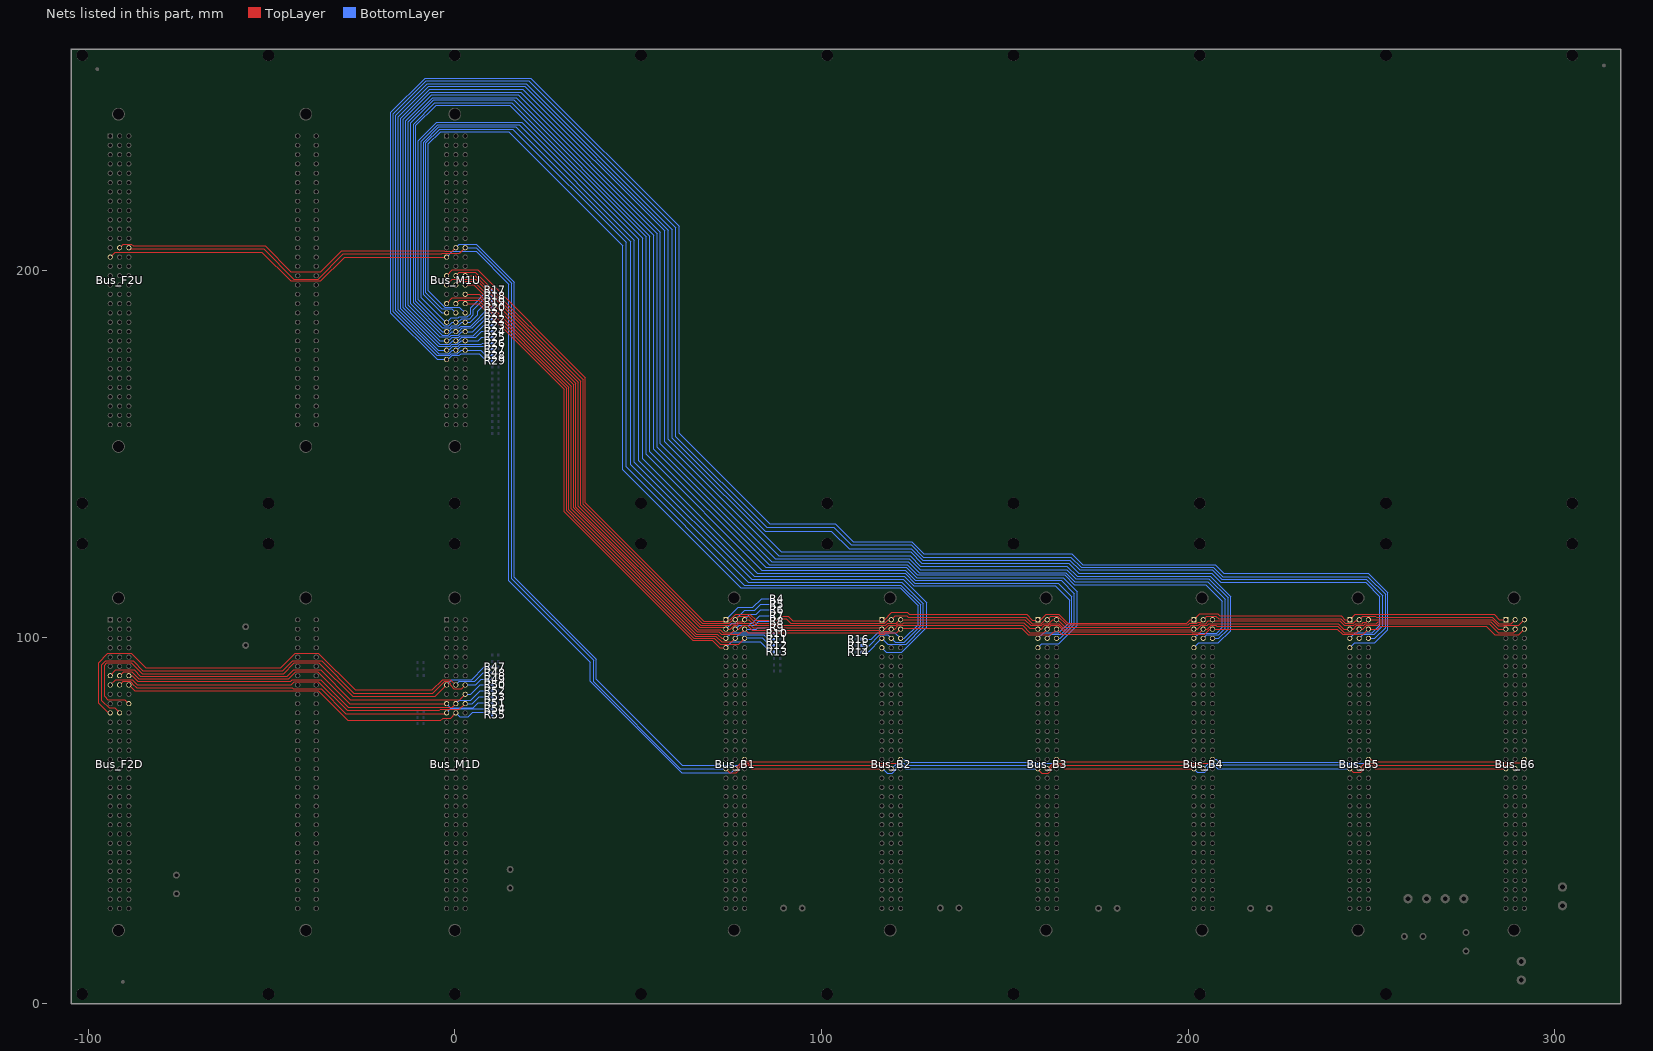
[diagram p0: the nets of this part, all layers, seen from the top]
# Altium PCB MISC67337.PcbDoc (part 6 of 7)
Units mm, origin at the board's own origin, x right, y up, seen from the top; angles counter-clockwise.
Board outline 422.71 x 260.35 mm, 4 copper layers (TopLayer, InternalPlane1, InternalPlane2, BottomLayer); 82 components, 143 nets, 1295 pads, 42 vias.

## Via types
v1: diameter 0.61, hole 0.305, TopLayer to BottomLayer, 42 vias

## Nets (pads, with @x,y where several pads share a name; then routed paths per layer and width w, separated by ;. In a path a pad name is that pad's centre, name@x,y a point inside that pad or via, vN(x,y) a via of type N, cw(c..) or ccw(c..) an arc to the next point about the centre after c; other vN are vias at no path point) (continued)
B_DSP2_XD13: Bus_B1.C16 Bus_B2.C16 Bus_B3.C16 Bus_B4.C16 Bus_B5.C16 Bus_B6.C16 Bus_F2U.B13 Bus_M1U.B13 | length 511.1
  TopLayer w0.254: Bus_F2U.B13@-91.388,206.173 Bus_F2U.B13@-91.43,206.173 -90.466,207.137 -90.272,207.137 -90.257,207.151 -88.203,207.151 -87.74,206.688 -54.813,206.688 ; -54.102,206.688 -54.813,206.688 ; -29.5,205.327 -28.956,205.327 ; Bus_M1U.B13@0.3,206.173 -0.678,205.196 -2.732,205.196 -2.863,205.327 -28.956,205.327 ; Bus_B1.C16@79.035,66.504 79.144,66.504 79.683,65.965 107.848,65.965 ; 110.425,65.965 107.848,65.965 ; Bus_B2.C16@121.585,66.613 120.504,65.532 115.773,65.532 115.34,65.965 107.848,65.965 ; Bus_B3.C16@164.13,66.613 165.01,66.613 165.653,65.97 200.476,65.97 200.889,65.557 ; 200.863,65.557 200.889,65.557 ; Bus_B4.C16@206.675,66.486 205.746,65.557 200.889,65.557 ; Bus_B5.C16@249.22,66.613 249.885,66.613 250.52,65.978 252.552,65.978 ; 251.079,65.978 252.552,65.978 ; 278.638,65.978 277.241,65.978 ; Bus_B6.C16@291.765,66.613 290.787,65.635 285.75,65.635 285.407,65.978 277.241,65.978 ; -54.813,206.688 -51.723,206.688 -44.679,199.644 -36.5,199.644 -30.817,205.327 -28.956,205.327 ; 252.552,65.978 277.241,65.978
  BottomLayer w0.254: Bus_M1U.B13@0.3,206.173 1.278,207.151 5.904,207.151 16.256,196.799 16.256,116.332 38.608,93.98 38.608,88.519 62.076,65.051 77.473,65.051 Bus_B1.C16@79.035,66.613 ; Bus_B2.C16@121.585,66.613 122.617,66.613 123.325,65.905 154.559,65.905 ; 154.813,65.905 154.559,65.905 ; Bus_B3.C16@164.257,66.675 163.176,65.594 160.833,65.594 160.807,65.619 158.318,65.619 158.033,65.905 154.559,65.905 ; Bus_B4.C16@206.675,66.613 207.631,66.613 208.347,65.897 210.947,65.897 ; 210.972,65.897 243.018,65.897 243.357,65.557 245.77,65.557 ; 245.796,65.532 248.139,65.532 Bus_B5.C16@249.22,66.613
B_DSP2_XD14: Bus_B1.A17 Bus_B2.A17 Bus_B3.A17 Bus_B4.A17 Bus_B5.A17 Bus_B6.A17 Bus_F2U.C13 Bus_M1U.C13 | length 508.7
  TopLayer w0.254: Bus_F2U.C13@-88.89,205.833 -53.823,205.833 ; -52.63,205.833 -53.823,205.833 ; -28.637,204.48 -26.518,204.48 ; 1.456,204.789 Bus_M1U.C13@2.84,206.173 1.278,204.611 -3.476,204.611 -3.607,204.48 -26.518,204.48 ; Bus_B1.A17@73.96,64.073 75.041,62.992 76.802,62.992 77.478,63.668 77.478,64.27 78.334,65.126 79.908,65.126 80.961,64.073 Bus_B2.A17@116.505,64.073 ; Bus_B3.A17@159.05,63.946 160.131,62.865 161.892,62.865 162.568,63.541 162.568,64.143 163.525,65.1 165.303,65.1 166.33,64.073 Bus_B4.A17@201.595,64.073 ; Bus_B5.A17@244.14,64.073 245.118,63.095 247.118,63.095 248.031,64.008 248.031,64.389 248.693,65.051 250.087,65.051 251.065,64.073 Bus_B6.A17@286.685,64.073 ; -53.823,205.833 -52.163,205.833 -43.942,197.612 -37.236,197.612 -30.368,204.48 -26.518,204.48
  BottomLayer w0.254: Bus_M1U.C13@2.84,206.173 2.892,206.121 5.893,206.121 15.494,196.52 15.494,115.951 37.846,93.599 37.846,87.757 61.53,64.073 Bus_B1.A17@73.955,64.073 ; Bus_B2.A17@116.632,64.135 117.902,62.865 119.318,62.865 120.396,63.943 120.396,64.451 121.058,65.113 121.933,65.113 122.973,64.073 127.686,64.073 ; 126.467,64.073 127.686,64.073 ; Bus_B3.A17@159.05,64.073 127.686,64.073 ; Bus_B3.A17@159.05,64.116 159.158,64.116 Bus_B3.A17@159.177,64.135 ; Bus_B4.A17@201.595,64.073 202.573,63.095 204.573,63.095 205.359,63.881 205.359,64.389 206.021,65.051 207.161,65.051 208.139,64.073 Bus_B5.A17@244.14,64.073 Bus_B5.A17@244.121,64.054
B_DSP2_XD15: Bus_B1.B17 Bus_B2.B17 Bus_B3.B17 Bus_B4.B17 Bus_B5.B17 Bus_B6.B17 Bus_F2U.A14 Bus_M1U.A14 | length 507.2
  TopLayer w0.254: Bus_F2U.A14@-93.97,203.633 -92.625,204.978 -52.578,204.978 -44.704,197.104 -36.525,197.104 -29.996,203.633 Bus_M1U.A14@-2.24,203.633 ; Bus_B1.B17@76.495,64.073 77.954,65.532 80.077,65.532 80.558,65.051 118.067,65.051 Bus_B2.B17@119.045,64.073 ; Bus_B3.B17@161.59,63.946 163.201,65.557 165.421,65.557 165.927,65.051 203.157,65.051 Bus_B4.B17@204.135,64.073 ; Bus_B4.B17@204.071,64.01 Bus_B4.B17@204.135,63.946 ; Bus_B5.B17@246.68,64.073 248.139,65.532 250.444,65.532 250.951,65.025 277.343,65.025 277.368,65.051 288.247,65.051 Bus_B6.B17@289.225,64.073
  BottomLayer w0.254: Bus_M1U.A14@-2.24,203.633 -0.678,205.196 5.802,205.196 14.732,196.266 14.732,115.316 36.957,93.091 36.957,87.884 61.849,62.992 75.414,62.992 Bus_B1.B17@76.495,64.073 ; Bus_B2.B17@119.172,64.135 120.631,65.594 122.442,65.594 123.047,64.989 154.788,64.989 ; 155.321,64.989 154.788,64.989 ; Bus_B3.B17@161.717,64.135 160.639,65.213 158.013,65.213 157.789,64.989 154.788,64.989 ; Bus_B4.B17@204.135,64.073 205.619,65.557 207.721,65.557 208.128,65.151 245.602,65.151 Bus_B5.B17@246.68,64.073
B_LZL1: Bus_F2D.B11 Bus_M1D.C8 R49.2 | length 132.2
  TopLayer w0.254: Bus_F2D.B11@-91.43,79.294 -92.781,80.645 -94.234,80.645 -96.266,82.677 -96.266,92.456 -95.25,93.472 -87.732,93.472 -85.09,90.83 -46.888,90.83 -44.247,93.472 -36.322,93.472 -27.483,84.633 -6.02,84.633 -2.761,87.892 -1.835,87.892 -1.262,87.319 -1.262,86.987 -0.211,85.936 1.862,85.936 Bus_M1D.C8@2.84,86.914
  BottomLayer w0.254: Bus_M1D.C8@2.84,86.914 5.71,86.914 7.29,88.494 R49.2@10.185,88.494
B_LZL2: Bus_F2D.A11 Bus_M1D.B8 R48.1 | length 134.4
  TopLayer w0.254: Bus_F2D.A11@-93.97,79.294 -94.534,79.294 -97.155,81.915 -97.155,92.964 -94.607,95.512 -88.29,95.512 -84.345,91.567 -47.523,91.567 -43.459,95.631 -37.186,95.631 -27.102,85.547 -6.096,85.547 -3.251,88.392 -1.178,88.392 Bus_M1D.B8@0.3,86.914
  BottomLayer w0.254: Bus_M1D.B8@0.3,86.914 1.278,87.892 5.444,87.892 7.747,90.195 R48.1@10.185,90.195
B_LZL3: Bus_F2D.C10 Bus_M1D.A8 R47.2 | length 131.5
  TopLayer w0.254: Bus_F2D.C10@-88.89,81.834 -89.987,82.931 -94.615,82.931 -95.504,83.82 -95.504,92.329 -94.861,92.972 -88.222,92.972 -85.293,90.043 -46.693,90.043 -43.764,92.972 -37.041,92.972 -27.864,83.795 -5.359,83.795 Bus_M1D.A8@-2.24,86.914
  BottomLayer w0.254: Bus_M1D.A8@-2.24,86.914 -0.762,88.392 4.674,88.392 8.103,91.821 R47.2@10.185,91.821
B_LZT1: Bus_F2D.C8 Bus_M1D.B11 R55.1 | length 105.1
  TopLayer w0.254: Bus_F2D.C8@-88.89,86.914 -87.32,85.344 -37.287,85.344 -29.235,77.292 -3.759,77.292 -3.2,77.851 -1.143,77.851 Bus_M1D.B11@0.3,79.294
  BottomLayer w0.254: Bus_M1D.B11@0.3,79.294 1.362,78.232 3.658,78.232 4.089,78.664 4.115,78.664 4.928,79.477 9.373,79.477 10.084,78.765 R55.1@10.185,78.765
B_LZT2: Bus_F2D.B8 Bus_M1D.A11 R54.2 | length 106.2
  TopLayer w0.254: Bus_F2D.B8@-91.43,86.914 -90.452,87.892 -88.485,87.892 -87.912,87.319 -87.912,87.302 -86.741,86.131 -44.323,86.131 -44.044,85.852 -36.449,85.852 -29.693,79.096 -2.764,79.096 -2.565,79.294 Bus_M1D.A11@-2.24,79.294
  BottomLayer w0.254: Bus_M1D.A11@-2.24,79.294 -1.168,80.366 10.16,80.366 R54.2@10.185,80.391
B_LZT3: Bus_F2D.A8 Bus_M1D.C10 R53.2 | length 110.5
  TopLayer w0.254: Bus_F2D.A8@-93.97,86.914 -92.492,88.392 -87.986,88.392 -86.614,87.02 -44.602,87.02 -43.794,87.828 -37.206,87.828 -29.337,79.959 -4.191,79.959 -3.878,80.272 1.278,80.272 Bus_M1D.C10@2.84,81.834
  BottomLayer w0.254: Bus_M1D.C10@2.84,81.834 4.77,81.834 6.629,83.693 R53.2@10.185,83.693
B_LZT4: Bus_F2D.C7 Bus_M1D.B10 R52.1 | length 104.9
  TopLayer w0.254: Bus_F2D.C7@-88.89,89.454 -88.006,89.454 -86.462,87.909 -44.78,87.909 -44.298,88.392 -36.525,88.392 -28.989,80.856 -0.678,80.856 Bus_M1D.B10@0.3,81.834
  BottomLayer w0.254: Bus_M1D.B10@0.3,81.834 1.278,82.812 4.351,82.812 6.934,85.395 R52.1@10.185,85.395
B_LZT5: Bus_F2D.B7 Bus_M1D.A10 R51.2 | length 108.2
  TopLayer w0.254: Bus_F2D.B7@-91.43,89.454 -90.333,90.551 -88.062,90.551 -86.157,88.646 -45.237,88.646 -43.332,90.551 -37.338,90.551 -28.621,81.834 Bus_M1D.A10@-2.24,81.834
  BottomLayer w0.254: Bus_M1D.A10@-2.24,81.834 -1.178,80.772 5.08,80.772 6.35,82.042 R51.2@10.185,82.042
B_LZT6: Bus_F2D.A7 Bus_M1D.C9 R50.2 | length 111.3
  TopLayer w0.254: Bus_F2D.A7@-93.97,89.454 -92.408,91.016 -87.435,91.016 -85.725,89.306 -45.677,89.306 -43.967,91.016 -36.609,91.016 -28.524,82.931 1.397,82.931 Bus_M1D.C9@2.84,84.374
  BottomLayer w0.254: Bus_M1D.C9@2.84,84.374 4.364,84.374 6.985,86.995 R50.2@10.185,86.995
B_ZL1: Bus_B1.A1 Bus_B2.A1 Bus_B3.A1 Bus_B4.A1 Bus_B5.A1 Bus_B6.A1 Bus_M1U.A16 R4.2 | length 373.7
  TopLayer w0.254: Bus_M1U.A16@-2.24,198.553 -0.678,200.116 6.234,200.116 35.636,170.713 35.636,136.652 67.945,104.343 73.585,104.343 Bus_B1.A1@73.955,104.713 75.112,104.713 76.673,106.274 80.467,106.274 82.169,104.572 87.808,104.572 88.9,105.664 90.907,105.664 92.202,104.369 116.161,104.369 Bus_B2.A1@116.505,104.713 117.235,104.713 119.253,106.731 123.419,106.731 123.977,106.172 156.007,106.172 157.556,104.623 158.96,104.623 Bus_B3.A1@159.05,104.713 159.882,104.713 161.392,106.223 164.744,106.223 167.183,103.784 199.72,103.784 200.649,104.713 Bus_B4.A1@201.595,104.713 203.206,106.324 208.051,106.324 208.636,105.74 241.783,105.74 242.81,104.713 Bus_B5.A1@244.14,104.713 245.624,106.197 283.464,106.197 284.948,104.713 Bus_B6.A1@286.685,104.713
  BottomLayer w0.254: Bus_B1.A1@73.955,104.713 77.319,108.077 81.28,108.077 83.693,110.49 R4.2@87.097,110.49
B_ZL2: Bus_B1.B1 Bus_B2.B1 Bus_B3.B1 Bus_B4.B1 Bus_B5.B1 Bus_B6.B1 Bus_M1U.B16 R5.1 | length 371.7
  TopLayer w0.254: Bus_M1U.B16@0.3,198.553 1.278,199.531 5.624,199.531 35.001,170.155 35.001,136.195 67.461,103.735 74.933,103.735 75.911,104.713 Bus_B1.B1@76.495,104.713 ; Bus_B1.B1@76.259,104.713 Bus_B1.B1@76.495,104.713 ; Bus_B6.B1@289.225,104.713 288.144,103.632 284.759,103.632 283.032,105.359 251.435,105.359 251.103,105.691 247.658,105.691 Bus_B5.B1@246.68,104.713 246.412,104.445 245.796,104.445 245.059,103.708 242.926,103.708 241.681,104.953 208.356,104.953 207.618,105.691 205.113,105.691 Bus_B4.B1@204.135,104.713 203.486,104.064 202.738,104.064 202.409,103.735 200.482,103.735 200.049,103.302 166.98,103.302 166.776,103.505 166.721,103.505 164.535,105.691 162.568,105.691 Bus_B3.B1@161.59,104.713 161.025,104.713 159.944,103.632 157.556,103.632 155.753,105.435 123.647,105.435 123.317,105.766 120.098,105.766 Bus_B2.B1@119.045,104.713 118.98,104.648 118.237,104.648 117.324,103.735 91.692,103.735 90.399,105.029 89.205,105.029 87.935,103.759 82.118,103.759 80.186,105.691 78.63,105.691 78.602,105.663 77.445,105.663 Bus_B1.B1@76.495,104.713
  BottomLayer w0.254: Bus_B1.B1@76.495,104.713 79.097,107.315 81.788,107.315 83.464,108.991 R5.1@87.097,108.991
B_ZL3: Bus_B1.C1 Bus_B2.C1 Bus_B3.C1 Bus_B4.C1 Bus_B5.C1 Bus_B6.C1 Bus_M1U.C16 R6.2 | length 364.6
  TopLayer w0.254: Bus_M1U.C16@2.84,198.553 5.57,198.553 34.366,169.757 34.366,135.932 67.098,103.2 75.26,103.2 75.717,103.657 76.823,103.657 77.307,104.142 78.464,104.142 Bus_B1.C1@79.035,104.713 80.25,104.713 81.788,103.175 117.499,103.175 118.059,103.735 120.366,103.735 121.344,104.713 Bus_B2.C1@121.585,104.713 155.51,104.713 157.072,103.151 160.149,103.151 160.655,103.657 162.011,103.657 163.066,104.713 Bus_B3.C1@164.13,104.713 164.527,104.713 166.548,102.692 200.457,102.692 200.916,103.151 202.821,103.151 203.327,103.657 204.775,103.657 205.511,104.394 241.376,104.394 242.595,103.175 245.262,103.175 245.77,103.683 247.472,103.683 247.828,104.038 248.545,104.038 Bus_B5.C1@249.22,104.713 283.018,104.713 284.605,103.126 286.256,103.126 286.28,103.151 290.203,103.151 Bus_B6.C1@291.765,104.713
  BottomLayer w0.254: Bus_B1.C1@79.035,104.713 80.494,106.172 82.169,106.172 83.439,107.442 R6.2@87.097,107.442
B_ZL4: Bus_B1.A2 Bus_B2.A2 Bus_B3.A2 Bus_B4.A2 Bus_B5.A2 Bus_B6.A2 Bus_M1U.A17 R7.2 | length 370.4
  TopLayer w0.254: Bus_M1U.A17@-2.24,196.013 -0.692,197.561 5.664,197.561 33.706,169.52 33.706,135.694 66.759,102.641 73.487,102.641 Bus_B1.A2@73.955,102.173 75.105,102.173 76.183,103.251 76.991,103.251 77.475,103.735 80.161,103.735 81.407,102.489 116.189,102.489 Bus_B2.A2@116.505,102.173 117.286,102.173 118.364,103.251 120.456,103.251 120.763,103.557 122.149,103.557 122.477,103.886 155.219,103.886 156.769,102.337 158.886,102.337 Bus_B3.A2@159.05,102.173 159.958,102.173 160.936,103.151 162.079,103.151 162.56,103.632 164.77,103.632 166.37,102.032 Bus_B4.A2@201.595,102.032 ; Bus_B4.A2@201.595,102.173 202.528,102.173 203.606,103.251 205.207,103.251 205.613,103.657 241.021,103.657 242.505,102.173 Bus_B5.A2@244.14,102.173 245.048,102.173 246.026,103.151 247.085,103.151 247.087,103.149 247.879,103.149 248.361,103.632 251.282,103.632 251.841,104.191 282.6,104.191 284.618,102.173 Bus_B6.A2@286.685,102.173
  BottomLayer w0.254: Bus_B1.A2@73.955,102.173 75.517,103.735 81.129,103.735 83.236,105.842 R7.2@87.097,105.842
B_ZL5: Bus_B1.B2 Bus_B2.B2 Bus_B3.B2 Bus_B4.B2 Bus_B5.B2 Bus_B6.B2 Bus_M1U.B17 R8.1 | length 370
  TopLayer w0.254: Bus_M1U.B17@0.3,196.013 1.278,196.991 5.243,196.991 33.045,169.189 33.045,135.457 66.47,102.032 72.39,102.032 73.227,101.195 75.517,101.195 Bus_B1.B2@76.495,102.173 77.408,102.173 78.486,103.251 79.756,103.251 81.178,101.829 115.466,101.829 116.1,101.195 116.91,101.195 117.34,101.625 118.497,101.625 Bus_B2.B2@119.045,102.173 119.953,102.173 120.931,103.151 154.888,103.151 156.843,101.195 160.612,101.195 Bus_B3.B2@161.59,102.173 161.736,102.173 162.714,103.151 164.565,103.151 166.294,101.422 200.963,101.422 201.19,101.195 203.157,101.195 Bus_B4.B2@204.135,102.173 205.292,102.173 206.27,103.151 207.542,103.151 207.797,102.895 240.894,102.895 242.594,101.195 245.848,101.195 246.826,102.173 247.715,102.173 248.693,103.151 251.792,103.151 252.222,103.581 282.219,103.581 284.605,101.195 288.901,101.195 289.966,102.26
  BottomLayer w0.254: Bus_B1.B2@76.495,102.173 77.573,103.251 81.915,103.251 82.906,104.242 R8.1@87.097,104.242
B_ZL6: Bus_B1.C2 Bus_B2.C2 Bus_B3.C2 Bus_B4.C2 Bus_B5.C2 Bus_B6.C2 Bus_M1U.C17 R9.2 | length 366.6
  TopLayer w0.254: Bus_M1U.C17@2.84,196.013 5.205,196.013 8.395,192.824 ; 6.425,194.794 8.395,192.824 ; Bus_B6.C2@291.765,102.173 290.203,100.611 283.691,100.611 281.407,102.895 252.425,102.895 251.703,102.173 Bus_B5.C2@249.22,102.173 247.733,100.686 242.164,100.686 240.676,102.173 Bus_B4.C2@206.675,102.173 205.957,102.173 204.572,100.787 165.516,100.787 Bus_B3.C2@164.13,102.173 162.568,100.611 156.386,100.611 154.584,102.413 121.825,102.413 120.555,101.143 117.432,101.143 117.078,100.789 115.932,100.789 115.578,101.143 80.065,101.143 Bus_B1.C2@79.035,102.173 77.548,100.686 72.669,100.686 71.958,101.397 66.207,101.397 32.41,135.194 32.41,168.808 8.395,192.824
  BottomLayer w0.254: Bus_B1.C2@79.035,102.173 82.234,102.173 82.626,102.565 R9.2@87.097,102.565
BZT1: Bus_B1.A3 Bus_M1U.C18 R10.2 | length 143.5
  TopLayer w0.254: Bus_M1U.C18@2.84,193.473 6.712,193.473 31.775,168.41 31.775,134.93 33.794,132.912 34.712,131.994 65.893,100.813 71.628,100.813 72.808,99.633 Bus_B1.A3@73.955,99.633
  BottomLayer w0.254: Bus_B1.A3@73.955,99.633 75.517,101.195 84.733,101.195 84.963,100.965 R10.2@87.097,100.965
BZT2: Bus_B1.B3 Bus_M1U.A19 R11.2 | length 149.8
  TopLayer w0.254: Bus_M1U.A19@-2.24,190.933 -0.692,192.481 6.806,192.481 31.14,168.147 31.14,134.667 34.502,131.306 65.579,100.228 71.247,100.228 72.82,98.655 75.517,98.655 Bus_B1.B3@76.495,99.633
  BottomLayer w0.254: Bus_B1.B3@76.495,99.633 77.473,100.611 84.301,100.611 85.522,99.39 R11.2@87.097,99.39
BZT3: Bus_B1.C3 Bus_M1U.B19 R12.1 | length 147.8
  TopLayer w0.254: Bus_M1U.B19@0.3,190.933 1.278,191.911 3.245,191.911 3.259,191.897 6.492,191.897 30.505,167.884 30.505,134.404 34.238,130.671 65.24,99.67 70.764,99.67 72.363,98.071 77.473,98.071 Bus_B1.C3@79.035,99.633
  BottomLayer w0.254: Bus_B1.C3@79.035,99.633 79.224,99.822 82.169,99.822 ; 82.55,99.822 82.169,99.822 ; R12.1@86.97,97.917 R12.1@87.097,97.79 85.852,97.79 83.82,99.822 82.169,99.822
BZT4: Bus_B1.A4 Bus_M1U.C19 R13.2 | length 144.5
  TopLayer w0.254: Bus_M1U.C19@2.84,190.933 6.558,190.933 29.87,167.621 29.87,134.141 64.876,99.136 70.256,99.136 72.3,97.093 Bus_B1.A4@73.955,97.093
  BottomLayer w0.254: Bus_B1.A4@73.955,97.093 75.517,98.655 83.336,98.655 86.055,95.936 R13.2@87.097,95.936
BZT5: Bus_B2.A3 Bus_M1U.A20 R14.2 | length 304.8
  BottomLayer w0.254: Bus_M1U.A20@-2.24,188.393 -3.507,188.393 -8.509,193.396 -8.509,235.008 -4.376,239.141 16.688,239.141 47.981,207.848 47.981,146.939 79.985,114.935 121.92,114.935 127.838,109.017 127.838,102.794 123.088,98.044 122.017,98.044 121.99,98.071 118.067,98.071 Bus_B2.A3@116.505,99.633 112.757,95.885 R14.2@111.049,95.885
BZT6: Bus_B2.B3 Bus_M1U.B20 R15.1 | length 303.2
  BottomLayer w0.254: Bus_M1U.B20@0.3,188.393 -0.856,189.549 -3.545,189.549 -7.874,193.878 -7.874,234.745 -4.113,238.506 15.875,238.506 46.736,207.645 46.736,146.38 78.943,114.173 121.691,114.173 127.127,108.737 127.127,103.048 122.631,98.552 120.126,98.552 Bus_B2.B3@119.045,99.633 118.067,100.611 115.978,100.611 113.03,97.663 R15.1@111.049,97.663
BZT7: Bus_B2.C3 Bus_M1U.C20 R16.2 | length 300.4
  BottomLayer w0.254: Bus_M1U.C20@2.84,188.393 1.278,189.956 -2.758,189.956 -7.239,194.437 -7.239,234.482 -3.85,237.871 14.681,237.871 45.822,206.731 45.822,145.567 77.978,113.411 121.488,113.411 126.365,108.534 126.365,103.378 122.62,99.633 Bus_B2.C3@121.585,99.633 120.023,101.195 115.419,101.195 113.665,99.441 R16.2@111.049,99.441
BZT8: Bus_B2.A4 Bus_M1U.A21 R17.2 | length 320.9
  BottomLayer w0.254: R17.2@10.262,194.666 9.119,194.666 4.318,189.865 4.318,188.214 3.429,187.325 1.27,187.325 1.016,187.071 -1.022,187.071 Bus_M1U.A21@-2.24,185.853 -2.44,185.853 -9.144,192.557 -9.144,235.271 -4.639,239.776 17.526,239.776 49.022,208.28 49.022,147.676 81.001,115.697 122.276,115.697 128.676,109.296 128.676,102.641 121.92,95.885 117.713,95.885 Bus_B2.A4@116.505,97.093
BZT9: Bus_B3.A3 Bus_M1U.B21 R18.1 | length 356.3
  BottomLayer w0.254: R18.1@10.262,193.065 8.915,193.065 5.073,189.223 5.073,187.84 4.064,186.831 1.862,186.831 0.884,185.853 Bus_M1U.B21@0.3,185.853 -0.71,185.853 -1.687,184.876 -2.808,184.876 -9.931,191.999 -9.931,235.382 -4.902,240.411 18.288,240.411 50.19,208.509 50.19,148.031 81.636,116.586 122.555,116.586 125.222,113.919 163.83,113.919 167.691,110.058 167.691,104.089 164.797,101.195 160.612,101.195 Bus_B3.A3@159.05,99.633
BZT10: Bus_B3.B3 Bus_M1U.C21 R19.2 | length 363
  BottomLayer w0.254: R19.2@10.262,191.491 8.865,191.491 6.223,188.849 6.223,187.833 4.243,185.853 Bus_M1U.C21@2.84,185.853 1.957,185.853 0.98,184.876 -0.798,184.876 -1.27,184.404 -3.429,184.404 -10.617,191.592 -10.617,239.522 -5.086,245.053 14.966,245.053 51.232,208.788 51.232,148.666 82.55,117.348 122.809,117.348 125.476,114.681 164.592,114.681 168.326,110.947 168.326,103.657 165.379,100.711 162.668,100.711 Bus_B3.B3@161.59,99.633
BZT11: Bus_B3.C3 Bus_M1U.A22 R20.2 | length 363.9
  BottomLayer w0.254: R20.2@10.262,189.916 9.449,189.916 4.318,184.785 1.778,184.785 1.284,184.291 -0.621,184.291 -1.599,183.313 Bus_M1U.A22@-2.24,183.313 -3.38,183.313 -11.252,191.186 -11.252,239.903 -5.41,245.745 15.545,245.745 52.172,209.118 52.172,149.784 83.718,118.237 122.809,118.237 125.603,115.443 165.354,115.443 168.961,111.836 168.961,103.48 165.114,99.633 Bus_B3.C3@164.13,99.633
BZT12: Bus_B3.A4 Bus_M1U.B22 R21.1 | length 374.3
  BottomLayer w0.254: R21.1@10.262,188.316 8.85,188.316 4.826,184.291 2.046,184.291 1.068,183.313 Bus_M1U.B22@0.3,183.313 -0.837,183.313 -1.814,182.336 -3.393,182.336 -11.963,190.906 -11.963,240.208 -5.664,246.507 16.104,246.507 53.238,209.372 53.238,150.546 84.785,118.999 123.088,118.999 125.984,116.103 165.964,116.103 169.748,112.319 169.748,103.175 164.744,98.171 160.128,98.171 Bus_B3.A4@159.05,97.093
BZT13: Bus_B4.A3 Bus_M1U.C22 R22.2 | length 410.5
  BottomLayer w0.254: R22.2@10.262,186.69 8.255,186.69 4.878,183.313 Bus_M1U.C22@2.84,183.313 1.957,183.313 0.98,182.336 -0.925,182.336 -1.397,181.864 -4.039,181.864 -12.649,190.475 -12.649,240.487 -5.994,247.142 16.815,247.142 54.331,209.626 54.331,151.155 85.725,119.761 123.368,119.761 126.213,116.916 166.319,116.916 168.935,114.3 204.851,114.3 209.347,109.804 209.347,102.667 207.772,101.092 203.054,101.092 Bus_B4.A3@201.595,99.633
BZT14: Bus_B4.B3 Bus_M1U.A23 R23.2 | length 412.5
  BottomLayer w0.254: R23.2@10.262,185.064 7.899,185.064 4.993,182.158 1.437,182.158 1.03,181.751 -0.621,181.751 -1.599,180.773 Bus_M1U.A23@-2.24,180.773 -4.04,180.773 -13.335,190.068 -13.335,240.817 -6.299,247.853 17.323,247.853 55.245,209.931 55.245,151.74 86.462,120.523 123.723,120.523 126.67,117.577 166.624,117.577 169.113,115.087 205.334,115.087 210.109,110.312 210.109,102.337 208.356,100.584 207.107,100.584 207.08,100.611 205.113,100.611 Bus_B4.B3@204.135,99.633
BZT15: Bus_B4.C3 Bus_M1U.B23 R24.1 | length 414.1
  BottomLayer w0.254: R24.1@10.262,183.388 7.366,183.388 5.729,181.751 1.919,181.751 0.941,180.773 Bus_M1U.B23@0.3,180.773 -0.583,180.773 -1.56,179.796 -4.078,179.796 -14.021,189.738 -14.021,241.173 -6.629,248.564 17.983,248.564 56.109,210.439 56.109,152.654 87.351,121.412 124.003,121.412 127.025,118.389 166.903,118.389 169.393,115.9 205.664,115.9 210.922,110.642 210.922,102.159 208.396,99.633 Bus_B4.C3@206.675,99.633
BZT16: Bus_B4.A4 Bus_M1U.C23 R25.2 | length 423.9
  BottomLayer w0.254: R25.2@10.262,181.762 7.391,181.762 6.402,180.773 Bus_M1U.C23@2.84,180.773 1.703,180.773 0.726,179.796 -0.798,179.796 -1.27,179.324 -4.445,179.324 -14.707,189.586 -14.707,241.529 -6.833,249.403 18.567,249.403 57.226,210.744 57.226,153.314 88.367,122.174 124.181,122.174 127,119.355 166.98,119.355 169.748,116.586 206.045,116.586 211.607,111.023 211.607,101.752 208.28,98.425 202.927,98.425 Bus_B4.A4@201.595,97.093
BZT17: Bus_B5.A3 Bus_M1U.A24 R26.2 | length 463.5
  BottomLayer w0.254: R26.2@10.262,180.162 7.569,180.162 7.203,179.796 1.361,179.796 0.889,179.324 -0.508,179.324 -1.599,178.233 Bus_M1U.A24@-2.24,178.233 -4.447,178.233 -15.418,189.205 -15.418,241.96 -7.137,250.241 19.025,250.241 58.268,210.998 58.268,153.949 89.027,123.19 124.358,123.19 127.406,120.142 167.513,120.142 170.231,117.424 206.426,117.424 208.915,114.935 248.412,114.935 252.349,110.998 252.349,103.251 250.215,101.117 245.624,101.117 Bus_B5.A3@244.14,99.633
BZT18: Bus_B5.B3 Bus_M1U.B24 R27.1 | length 467.4
  BottomLayer w0.254: 8.382,179.324 6.731,179.324 ; R27.1@10.262,178.537 9.423,178.537 8.636,179.324 6.731,179.324 ; Bus_B5.B3@246.68,99.633 247.758,100.711 250.787,100.711 253.111,103.035 253.111,111.252 248.666,115.697 209.245,115.697 206.654,118.288 170.409,118.288 167.716,120.98 127.635,120.98 124.536,124.079 107.569,124.079 102.743,128.905 84.734,128.905 59.385,154.254 59.385,211.023 19.456,250.952 -7.518,250.952 -16.104,242.367 -16.104,188.951 -4.409,177.256 -1.687,177.256 -0.71,178.233 Bus_M1U.B24@0.3,178.233 0.56,178.233 1.651,179.324 6.731,179.324
BZT19: Bus_B5.C3 Bus_M1U.C24 R28.2 | length 467.8
  BottomLayer w0.254: R28.2@10.262,176.886 8.407,176.886 7.06,178.233 Bus_M1U.C24@2.84,178.233 1.703,178.233 0.726,177.256 -0.925,177.256 -1.397,176.784 -4.851,176.784 -16.739,188.671 -16.739,242.748 -7.772,251.714 20.193,251.714 60.274,211.633 60.274,154.686 85.039,129.921 103.378,129.921 108.204,125.095 124.536,125.095 127.838,121.793 168.072,121.793 170.84,119.024 206.858,119.024 209.423,116.459 249.047,116.459 253.873,111.633 253.873,102.527 250.979,99.633 Bus_B5.C3@249.22,99.633
BZT20: Bus_B5.A4 Bus_M1U.A25 R29.2 | length 478.6
  BottomLayer w0.254: R29.2@10.262,175.311 8.585,175.311 6.64,177.256 1.742,177.256 1.27,176.784 -0.635,176.784 -1.726,175.693 Bus_M1U.A25@-2.24,175.693 -4.802,175.693 -17.424,188.316 -17.424,243.078 -8.052,252.451 20.752,252.451 61.214,211.988 61.214,155.6 85.877,130.937 103.759,130.937 108.712,125.984 124.689,125.984 127.94,122.733 168.275,122.733 171.247,119.761 207.366,119.761 209.779,117.348 249.225,117.348 254.508,112.065 254.508,101.981 250.952,98.425 245.472,98.425 Bus_B5.A4@244.14,97.093